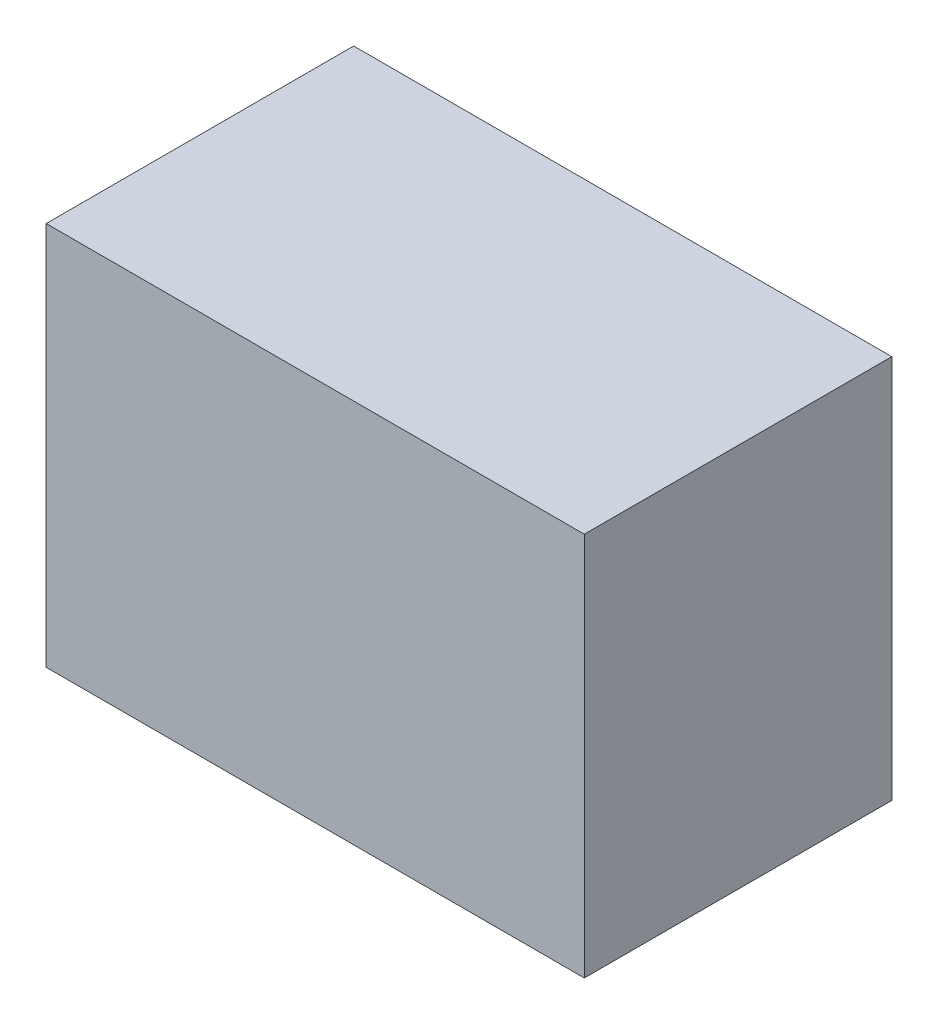
SolidWorks part; units mm, degrees
ref_plane "前视基准面" through (0, 0, 0) normal (0, 0, 1) x (1, 0, 0)
ref_plane "上视基准面" through (0, 0, 0) normal (0, 1, 0) x (1, 0, 0)
ref_plane "右视基准面" through (0, 0, 0) normal (1, 0, 0) x (0, 0, -1)
other "Configuration Table"
sketch "草图1" plane through (0, 0, 0) normal (0, 0, 1) x (1, 0, 0)
  line L0 (-14, -10) -> (14, -10)
  line L1 (14, -10) -> (14, 10)
  line L2 (14, 10) -> (-14, 10)
  line L3 (-14, 10) -> (-14, -10)
  point P0 (0, 0)
  dimension "D1" = 14
  dimension "D2" = 28
  dimension "D3" = 10
  dimension "D4" = 20
extrude "凸台-拉伸1" add sketch "草图1" against normal mid plane 16
